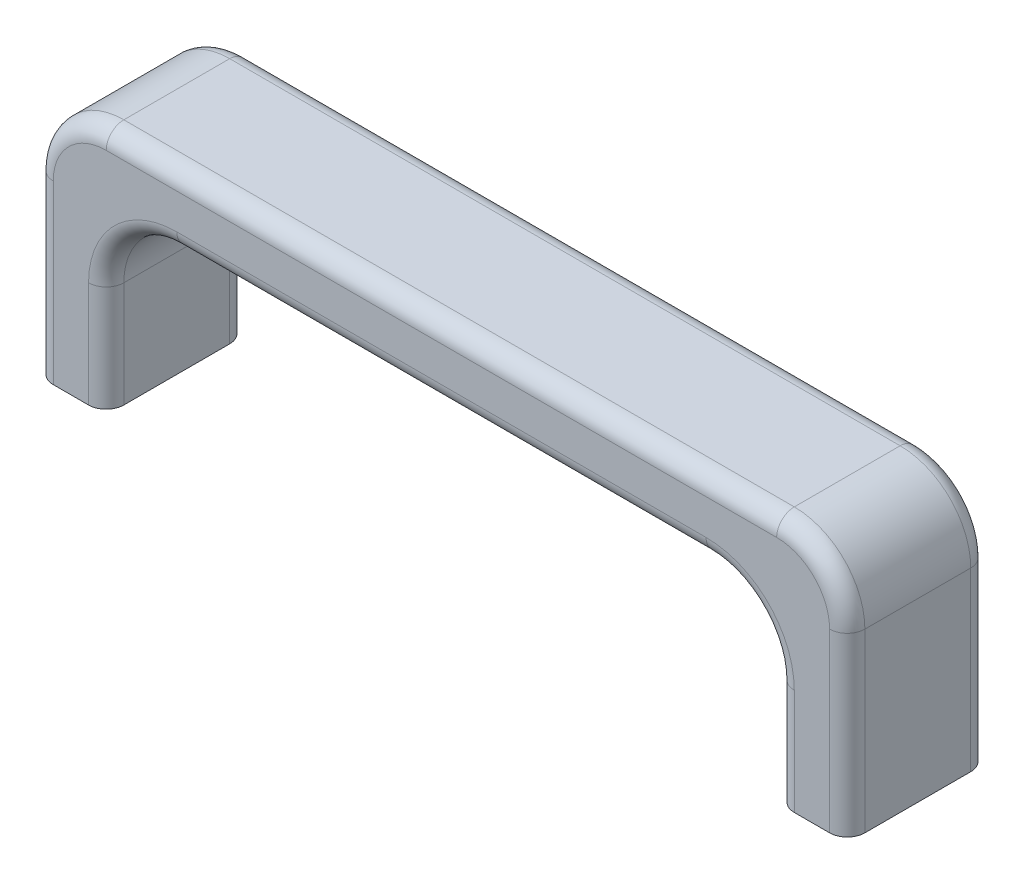
from build123d import *

# Parameters (mm, degrees)
BOSS_EXTRUDE1_DEPTH          = 20
FILLET1_R                    = 20
FILLET2_R                    = 5
M10_TAPPED_HOLE1_D           = 8.5
M10_TAPPED_HOLE1_DEPTH       = 25
M10_TAPPED_HOLE1_CSINK_D     = 10.05
M10_TAPPED_HOLE1_CSINK_ANGLE = 90
M10_TAPPED_HOLE1_TIP         = 2.553657631


with BuildPart() as part:
    # Sketch1 → Boss-Extrude1 (new, symmetric)
    with BuildSketch(Plane.XY):
        Polygon((-41, 226), (-41, 296), (189, 296), (189, 226), (169, 226), (169, 276), (-21, 276), (-21, 226), align=None)
    extrude(amount=BOSS_EXTRUDE1_DEPTH, both=True)

    # Fillet1
    fillet1_edges = [part.edges().sort_by_distance(p)[0] for p in [
        (-21, 276, 0),
        (169, 276, 0),
        (189, 296, 0),
        (-41, 296, 0),
    ]]
    fillet(fillet1_edges, radius=FILLET1_R)

    # Fillet2
    fillet2_edges = [part.edges().sort_by_distance(p)[0] for p in [
        (-41, 251, -20),
        (74, 296, -20),
        (74, 296, 20),
        (189, 251, -20),
        (169, 241, -20),
        (74, 276, -20),
        (-35.142135624, 290.142135624, -20),
        (183.142135624, 290.142135624, -20),
        (189, 251, 20),
        (74, 276, 20),
        (169, 241, 20),
        (-21, 241, 20),
        (-35.142135624, 290.142135624, 20),
        (183.142135624, 290.142135624, 20),
        (163.142135624, 270.142135624, -20),
        (163.142135624, 270.142135624, 20),
        (-15.142135624, 270.142135624, -20),
        (-15.142135624, 270.142135624, 20),
        (-21, 241, -20),
        (-41, 251, 20),
    ]]
    fillet(fillet2_edges, radius=FILLET2_R)

    # M10 Tapped Hole1
    with Locations(Plane(origin=(-31, 226, 0), x_dir=(0, 0, -1), z_dir=(0, -1, 0))):
        with Locations((0, 0), (0, 210)):
            CounterSinkHole(M10_TAPPED_HOLE1_D / 2, M10_TAPPED_HOLE1_CSINK_D / 2, depth=M10_TAPPED_HOLE1_DEPTH, counter_sink_angle=M10_TAPPED_HOLE1_CSINK_ANGLE)
            with Locations((0, 0, -(M10_TAPPED_HOLE1_DEPTH + M10_TAPPED_HOLE1_TIP / 2))):  # 118° drill point
                Cone(0, M10_TAPPED_HOLE1_D / 2, M10_TAPPED_HOLE1_TIP, mode=Mode.SUBTRACT)


solid = part.part
